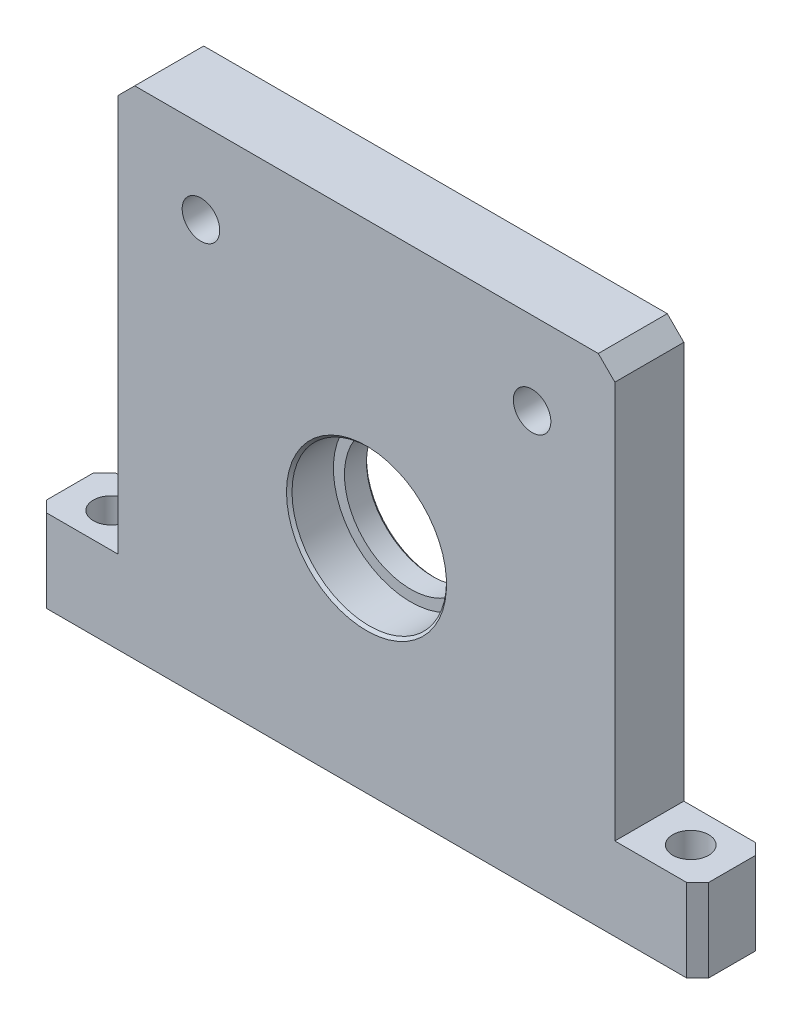
from build123d import *

# Parameters (mm, degrees)
SKETCH_1_W              = 12.5
SKETCH_1_H              = 90
EXTRUDE_1_DEPTH         = 90
CHAMFER_1_SIZE          = 3
HOLE_WIZARD_M8_1_D      = 6.8
SKETCH_6_R              = 14
CUT_EXTRUDE_1_DEPTH     = 8
SKETCH_7_R              = 12
CUT_EXTRUDE_2_DEPTH     = 128.530388535
CHAMFER_2_SIZE          = 0.5
SKETCH_10_W             = 12.5
SKETCH_10_H             = 15
EXTRUDE_3_DEPTH         = 15
SKETCH_11_W             = 12.5
SKETCH_11_H             = 15
EXTRUDE_4_DEPTH         = 15
CHAMFER_4_SIZE          = 2
HOLE_WIZARD_6_5_6_5_1_D = 6.5


with BuildPart() as part:
    # 草图1 → 凸台-拉伸1 (new body)
    with BuildSketch(Plane(origin=(0, 0, 0), x_dir=(0, 0, -1), z_dir=(1, 0, 0))):
        with Locations((6.25, 45)):
            Rectangle(SKETCH_1_W, SKETCH_1_H)
    extrude(amount=EXTRUDE_1_DEPTH)

    # 倒角1
    chamfer_1_edges = [part.edges().sort_by_distance(p)[0] for p in [
        (90, 90, -6.25),
        (0, 90, -6.25),
    ]]
    chamfer(chamfer_1_edges, length=CHAMFER_1_SIZE)

    # M8 螺纹孔1 (through all)
    with Locations(Plane(origin=(0, 0, -12.5), x_dir=(-1, 0, 0), z_dir=(0, 0, -1))):
        with Locations((-15, 75), (-75, 75)):
            Hole(HOLE_WIZARD_M8_1_D / 2)

    # 草图6 → 切除-拉伸1 (cut)
    with BuildSketch(Plane.XY):
        with Locations((45, 40)):
            Circle(SKETCH_6_R)
    extrude(amount=-CUT_EXTRUDE_1_DEPTH, mode=Mode.SUBTRACT)

    # 草图7 → 切除-拉伸2 (cut, through all)
    with BuildSketch(Plane.XY.offset(-8)):
        with Locations((45, 40)):
            Circle(SKETCH_7_R)
    extrude(amount=-CUT_EXTRUDE_2_DEPTH, mode=Mode.SUBTRACT)

    # 倒角2
    chamfer_2_edges = [part.edges().sort_by_distance(p)[0] for p in [
        (31, 40, 0),
        (33, 40, -12.5),
    ]]
    chamfer(chamfer_2_edges, length=CHAMFER_2_SIZE)

    # 草图10 → 凸台-拉伸3 (add)
    with BuildSketch(Plane(origin=(90, 0, 0), x_dir=(0, 0, -1), z_dir=(1, 0, 0))):
        with Locations((6.25, 7.5)):
            Rectangle(SKETCH_10_W, SKETCH_10_H)
    extrude(amount=EXTRUDE_3_DEPTH)

    # 草图11 → 凸台-拉伸4 (add)
    with BuildSketch(Plane.ZY):
        with Locations((-6.25, 7.5)):
            Rectangle(SKETCH_11_W, SKETCH_11_H)
    extrude(amount=EXTRUDE_4_DEPTH)

    # 倒角4
    chamfer_4_edges = [part.edges().sort_by_distance(p)[0] for p in [
        (105, 7.5, 0),
        (-15, 7.5, 0),
        (-15, 7.5, -12.5),
        (105, 7.5, -12.5),
    ]]
    chamfer(chamfer_4_edges, length=CHAMFER_4_SIZE)

    # Ø6.5 (6.5) 直径孔1 (through all)
    with Locations(Plane(origin=(-61.758148559, 15, 1.949959902), x_dir=(1, 0, 0), z_dir=(0, 1, 0))):
        with Locations((159.258148559, 8.199959902), (54.258148559, 8.199959902)):
            Hole(HOLE_WIZARD_6_5_6_5_1_D / 2)


solid = part.part
